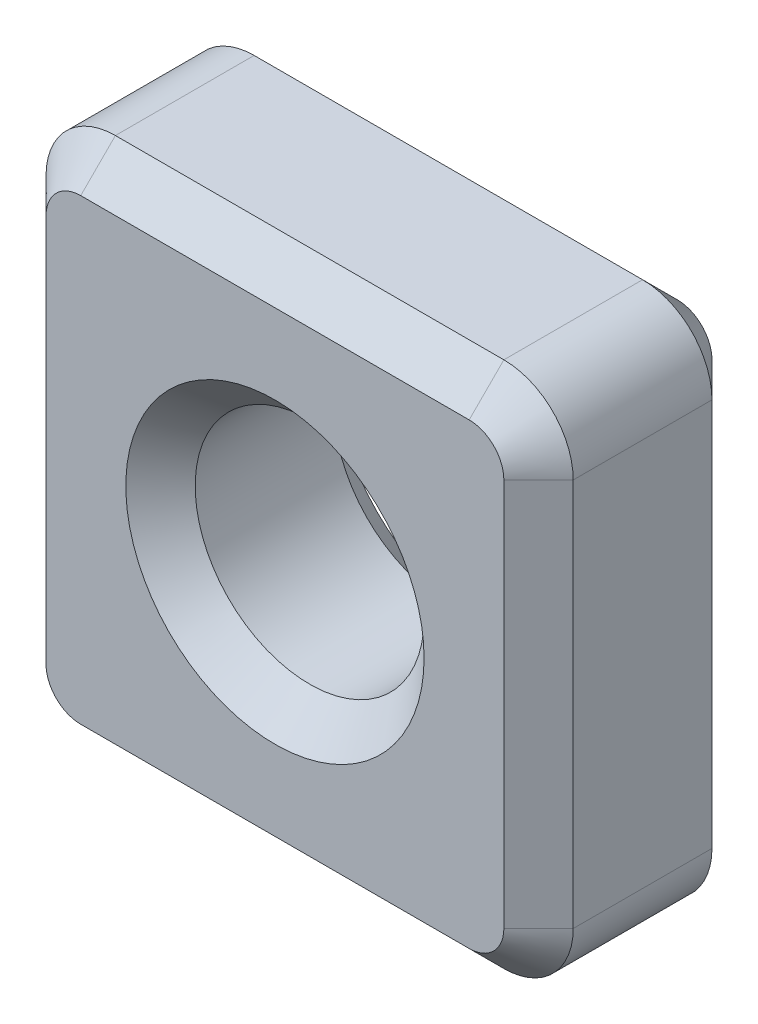
from build123d import *

# Parameters (mm, degrees)
SKETCH1_R             = 1.5
BOSS_EXTRUDE1_DEPTH   = 3
M4_TAPPED_HOLE1_D     = 3.3
M4_TAPPED_HOLE1_DEPTH = 11.5
M4_TAPPED_HOLE1_TIP   = 0.991420021
CHAMFER1_SIZE         = 0.5
CHAMFER2_SIZE         = 0.5
CHAMFER3_SIZE         = 0.5


with BuildPart() as part:
    # Sketch1 → Boss-Extrude1 (new body)
    with BuildSketch(Plane.XY):
        with BuildLine():
            Line((-2.8, 3.8), (2.8, 3.8))
            ThreePointArc((2.8, 3.8), (3.507106781, 3.507106781), (3.8, 2.8))
            Line((3.8, 2.8), (3.8, -2.8))
            ThreePointArc((3.8, -2.8), (3.507106781, -3.507106781), (2.8, -3.8))
            Line((2.8, -3.8), (-2.8, -3.8))
            ThreePointArc((-2.8, -3.8), (-3.507106781, -3.507106781), (-3.8, -2.8))
            Line((-3.8, -2.8), (-3.8, 2.8))
            ThreePointArc((-3.8, 2.8), (-3.507106781, 3.507106781), (-2.8, 3.8))
        make_face()
        Circle(SKETCH1_R, mode=Mode.SUBTRACT)
    extrude(amount=BOSS_EXTRUDE1_DEPTH)

    # M4 Tapped Hole1
    with Locations(Plane(origin=(0, 0, 0), x_dir=(-1, 0, 0), z_dir=(0, 0, -1))):
        with Locations((0, 0)):
            Hole(M4_TAPPED_HOLE1_D / 2, depth=M4_TAPPED_HOLE1_DEPTH)
            with Locations((0, 0, -(M4_TAPPED_HOLE1_DEPTH + M4_TAPPED_HOLE1_TIP / 2))):  # 118° drill point
                Cone(0, M4_TAPPED_HOLE1_D / 2, M4_TAPPED_HOLE1_TIP, mode=Mode.SUBTRACT)

    # Chamfer1
    chamfer1_edges = [part.edges().sort_by_distance(p)[0] for p in [
        (-1.65, 0, 0),
    ]]
    chamfer(chamfer1_edges, length=CHAMFER1_SIZE)

    # Chamfer2
    chamfer2_edges = [part.edges().sort_by_distance(p)[0] for p in [
        (-1.65, 0, 3),
    ]]
    chamfer(chamfer2_edges, length=CHAMFER2_SIZE)

    # Chamfer3
    chamfer3_edges = [part.edges().sort_by_distance(p)[0] for p in [
        (3.507106781, -3.507106781, 3),
        (0, -3.8, 0),
        (-3.507106781, -3.507106781, 0),
        (3.8, 0, 3),
        (3.507106781, 3.507106781, 3),
        (0, 3.8, 3),
        (-3.507106781, 3.507106781, 3),
        (-3.8, 0, 3),
        (-3.507106781, -3.507106781, 3),
        (0, -3.8, 3),
        (-3.8, 0, 0),
        (-3.507106781, 3.507106781, 0),
        (0, 3.8, 0),
        (3.507106781, 3.507106781, 0),
        (3.8, 0, 0),
        (3.507106781, -3.507106781, 0),
    ]]
    chamfer(chamfer3_edges, length=CHAMFER3_SIZE)


solid = part.part
